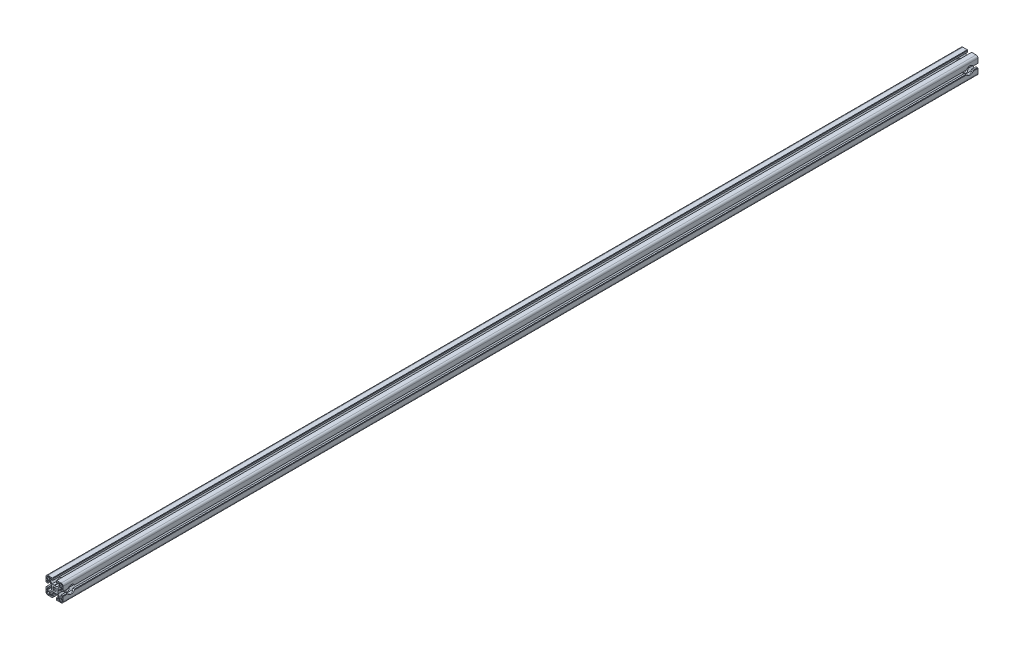
from build123d import *

# Parameters (mm, degrees)
EXTRUDE_1_DEPTH         = 2144
HOLE_WIZARD_19_0_19_1_D = 19


with BuildPart() as part:
    # 草图1 → 凸台-拉伸1 (new body)
    with BuildSketch(Plane.XY):
        with BuildLine():
            Line((-18.9995, -4.100341675), (-18.9995, -5.100341675))
            Line((-18.9995, -5.100341675), (-19.9995, -5.100341675))
            Line((-19.9995, -5.100341675), (-19.9995, -15.500341675))
            ThreePointArc((-19.9995, -15.500341675), (-18.681480515, -18.682322191), (-15.4995, -20.000341675))
            Line((-15.4995, -20.000341675), (-5.0995, -20.000341675))
            Line((-5.0995, -20.000341675), (-5.0995, -19.000341675))
            Line((-5.0995, -19.000341675), (-4.0995, -19.000341675))
            Line((-4.0995, -19.000341675), (-4.0995, -15.500341675))
            Line((-4.0995, -15.500341675), (-6.5995, -15.500341675))
            Line((-6.5995, -15.500341675), (-6.5995, -16.500341675))
            ThreePointArc((-6.5995, -16.500341675), (-6.892393219, -17.207448457), (-7.5995, -17.500341675))
            Line((-7.5995, -17.500341675), (-9.7995, -17.500341675))
            ThreePointArc((-9.7995, -17.500341675), (-10.153053391, -17.353895066), (-10.2995, -17.000341675))
            Line((-10.2995, -17.000341675), (-10.2995, -11.997341675))
            Line((-10.2995, -11.997341675), (-5.9025, -7.600341675))
            Line((-5.9025, -7.600341675), (-0.5195, -7.600341675))
            Line((-0.5195, -7.600341675), (0.0005, -7.300341675))
            Line((0.0005, -7.300341675), (0.5195, -7.600341675))
            Line((0.5195, -7.600341675), (5.9035, -7.600341675))
            Line((5.9035, -7.600341675), (10.3005, -11.997341675))
            Line((10.3005, -11.997341675), (10.3005, -17.000341675))
            ThreePointArc((10.3005, -17.000341675), (10.154053391, -17.353895066), (9.8005, -17.500341675))
            Line((9.8005, -17.500341675), (7.6005, -17.500341675))
            ThreePointArc((7.6005, -17.500341675), (6.893393219, -17.207448457), (6.6005, -16.500341675))
            Line((6.6005, -16.500341675), (6.6005, -15.500341675))
            Line((6.6005, -15.500341675), (4.1005, -15.500341675))
            Line((4.1005, -15.500341675), (4.1005, -19.000341675))
            Line((4.1005, -19.000341675), (5.1005, -19.000341675))
            Line((5.1005, -19.000341675), (5.1005, -20.000341675))
            Line((5.1005, -20.000341675), (15.5005, -20.000341675))
            ThreePointArc((15.5005, -20.000341675), (18.682480515, -18.682322191), (20.0005, -15.500341675))
            Line((20.0005, -15.500341675), (20.0005, -5.100341675))
            Line((20.0005, -5.100341675), (19.0005, -5.100341675))
            Line((19.0005, -5.100341675), (19.0005, -4.100341675))
            Line((19.0005, -4.100341675), (15.5005, -4.100341675))
            Line((15.5005, -4.100341675), (15.5005, -6.600341675))
            Line((15.5005, -6.600341675), (16.5005, -6.600341675))
            ThreePointArc((16.5005, -6.600341675), (17.207606781, -6.893234894), (17.5005, -7.600341675))
            Line((17.5005, -7.600341675), (17.5005, -9.800341675))
            ThreePointArc((17.5005, -9.800341675), (17.354053391, -10.153895066), (17.0005, -10.300341675))
            Line((17.0005, -10.300341675), (11.9975, -10.300341675))
            Line((11.9975, -10.300341675), (7.6005, -5.903341675))
            Line((7.6005, -5.903341675), (7.6005, -0.520341675))
            Line((7.6005, -0.520341675), (7.3005, -0.000341675))
            Line((7.3005, -0.000341675), (7.6005, 0.519658325))
            Line((7.6005, 0.519658325), (7.6005, 5.902658325))
            Line((7.6005, 5.902658325), (11.9975, 10.299658325))
            Line((11.9975, 10.299658325), (17.0005, 10.299658325))
            ThreePointArc((17.0005, 10.299658325), (17.354053391, 10.153211715), (17.5005, 9.799658325))
            Line((17.5005, 9.799658325), (17.5005, 7.599658325))
            ThreePointArc((17.5005, 7.599658325), (17.207606781, 6.892551543), (16.5005, 6.599658325))
            Line((16.5005, 6.599658325), (15.5005, 6.599658325))
            Line((15.5005, 6.599658325), (15.5005, 4.099658325))
            Line((15.5005, 4.099658325), (19.0005, 4.099658325))
            Line((19.0005, 4.099658325), (19.0005, 5.099658325))
            Line((19.0005, 5.099658325), (20.0005, 5.099658325))
            Line((20.0005, 5.099658325), (20.0005, 15.499658325))
            ThreePointArc((20.0005, 15.499658325), (18.682480515, 18.68163884), (15.5005, 19.999658325))
            Line((15.5005, 19.999658325), (5.1005, 19.999658325))
            Line((5.1005, 19.999658325), (5.1005, 18.999658325))
            Line((5.1005, 18.999658325), (4.1005, 18.999658325))
            Line((4.1005, 18.999658325), (4.1005, 15.499658325))
            Line((4.1005, 15.499658325), (6.6005, 15.499658325))
            ThreePointArc((6.6005, 15.499658325), (6.393348977, 15.999658325), (6.6005, 16.499658325))
            ThreePointArc((6.6005, 16.499658325), (6.893393219, 17.206765106), (7.6005, 17.499658325))
            Line((7.6005, 17.499658325), (9.8005, 17.499658325))
            ThreePointArc((9.8005, 17.499658325), (10.154053391, 17.353211715), (10.3005, 16.999658325))
            Line((10.3005, 16.999658325), (10.3005, 11.996658325))
            Line((10.3005, 11.996658325), (5.9035, 7.599658325))
            Line((5.9035, 7.599658325), (0.5195, 7.599658325))
            Line((0.5195, 7.599658325), (0.0005, 7.299658325))
            Line((0.0005, 7.299658325), (-0.5195, 7.599658325))
            Line((-0.5195, 7.599658325), (-5.9025, 7.599658325))
            Line((-5.9025, 7.599658325), (-10.2995, 11.996658325))
            Line((-10.2995, 11.996658325), (-10.2995, 16.999658325))
            ThreePointArc((-10.2995, 16.999658325), (-10.153053391, 17.353211715), (-9.7995, 17.499658325))
            Line((-9.7995, 17.499658325), (-7.5995, 17.499658325))
            ThreePointArc((-7.5995, 17.499658325), (-6.892393219, 17.206765106), (-6.5995, 16.499658325))
            Line((-6.5995, 16.499658325), (-6.5995, 15.499658325))
            Line((-6.5995, 15.499658325), (-4.0995, 15.499658325))
            Line((-4.0995, 15.499658325), (-4.0995, 18.999658325))
            Line((-4.0995, 18.999658325), (-5.0995, 18.999658325))
            Line((-5.0995, 18.999658325), (-5.0995, 19.999658325))
            Line((-5.0995, 19.999658325), (-15.4995, 19.999658325))
            ThreePointArc((-15.4995, 19.999658325), (-18.681480515, 18.68163884), (-19.9995, 15.499658325))
            Line((-19.9995, 15.499658325), (-19.9995, 5.099658325))
            Line((-19.9995, 5.099658325), (-18.9995, 5.099658325))
            Line((-18.9995, 5.099658325), (-18.9995, 4.099658325))
            Line((-18.9995, 4.099658325), (-15.4995, 4.099658325))
            Line((-15.4995, 4.099658325), (-15.4995, 6.599658325))
            Line((-15.4995, 6.599658325), (-16.4995, 6.599658325))
            ThreePointArc((-16.4995, 6.599658325), (-17.206606781, 6.892551543), (-17.4995, 7.599658325))
            Line((-17.4995, 7.599658325), (-17.4995, 9.799658325))
            ThreePointArc((-17.4995, 9.799658325), (-17.353053391, 10.153211715), (-16.9995, 10.299658325))
            Line((-16.9995, 10.299658325), (-11.9965, 10.299658325))
            Line((-11.9965, 10.299658325), (-7.5995, 5.902658325))
            Line((-7.5995, 5.902658325), (-7.5995, 0.519658325))
            Line((-7.5995, 0.519658325), (-7.2995, -0.000341675))
            Line((-7.2995, -0.000341675), (-7.5995, -0.520341675))
            Line((-7.5995, -0.520341675), (-7.5995, -5.903341675))
            Line((-7.5995, -5.903341675), (-11.9965, -10.300341675))
            Line((-11.9965, -10.300341675), (-16.9995, -10.300341675))
            ThreePointArc((-16.9995, -10.300341675), (-17.353053391, -10.153895066), (-17.4995, -9.800341675))
            Line((-17.4995, -9.800341675), (-17.4995, -7.600341675))
            ThreePointArc((-17.4995, -7.600341675), (-17.206606781, -6.893234894), (-16.4995, -6.600341675))
            Line((-16.4995, -6.600341675), (-15.4995, -6.600341675))
            Line((-15.4995, -6.600341675), (-15.4995, -4.100341675))
            Line((-15.4995, -4.100341675), (-18.9995, -4.100341675))
        make_face()
        with BuildLine():
            Line((15.5005, -18.000341675), (11.8005, -18.000341675))
            Line((11.8005, -18.000341675), (11.8005, -11.800341675))
            Line((11.8005, -11.800341675), (18.0005, -11.800341675))
            Line((18.0005, -11.800341675), (18.0005, -15.500341675))
            ThreePointArc((18.0005, -15.500341675), (17.268266953, -17.268108628), (15.5005, -18.000341675))
        make_face(mode=Mode.SUBTRACT)
        with BuildLine():
            Line((18.0005, 11.799658325), (11.8005, 11.799658325))
            Line((11.8005, 11.799658325), (11.8005, 17.999658325))
            Line((11.8005, 17.999658325), (15.5005, 17.999658325))
            ThreePointArc((15.5005, 17.999658325), (17.268266953, 17.267425278), (18.0005, 15.499658325))
            Line((18.0005, 15.499658325), (18.0005, 11.799658325))
        make_face(mode=Mode.SUBTRACT)
        with BuildLine():
            Line((-1.8145, -2.875341675), (-3.004391671, -4.066450004))
            Line((-3.004391671, -4.066450004), (-4.065608329, -3.005233346))
            Line((-4.065608329, -3.005233346), (-2.8745, -1.815341675))
            ThreePointArc((-2.8745, -1.815341675), (-3.399473913, -0.000341675), (-2.8745, 1.814658325))
            Line((-2.8745, 1.814658325), (-4.064391671, 3.005766654))
            Line((-4.064391671, 3.005766654), (-3.004391671, 4.065766654))
            Line((-3.004391671, 4.065766654), (-1.8145, 2.874658325))
            ThreePointArc((-1.8145, 2.874658325), (0, 3.399316649), (1.8145, 2.874658325))
            Line((1.8145, 2.874658325), (3.0055, 4.065658325))
            Line((3.0055, 4.065658325), (4.066608329, 3.004549996))
            Line((4.066608329, 3.004549996), (2.8755, 1.814658325))
            ThreePointArc((2.8755, 1.814658325), (3.400473913, -0.000341675), (2.8755, -1.815341675))
            Line((2.8755, -1.815341675), (4.066608329, -3.005233346))
            Line((4.066608329, -3.005233346), (3.0055, -4.066341675))
            Line((3.0055, -4.066341675), (1.8145, -2.875341675))
            ThreePointArc((1.8145, -2.875341675), (0, -3.4), (-1.8145, -2.875341675))
        make_face(mode=Mode.SUBTRACT)
        with BuildLine():
            Line((-17.9995, -15.500341675), (-17.9995, -11.800341675))
            Line((-17.9995, -11.800341675), (-11.7995, -11.800341675))
            Line((-11.7995, -11.800341675), (-11.7995, -18.000341675))
            Line((-11.7995, -18.000341675), (-15.4995, -18.000341675))
            ThreePointArc((-15.4995, -18.000341675), (-17.267266953, -17.268108628), (-17.9995, -15.500341675))
        make_face(mode=Mode.SUBTRACT)
        with BuildLine():
            Line((-11.7995, 17.999658325), (-11.7995, 11.799658325))
            Line((-11.7995, 11.799658325), (-17.9995, 11.799658325))
            Line((-17.9995, 11.799658325), (-17.9995, 15.499658325))
            ThreePointArc((-17.9995, 15.499658325), (-17.267266953, 17.267425278), (-15.4995, 17.999658325))
            Line((-15.4995, 17.999658325), (-11.7995, 17.999658325))
        make_face(mode=Mode.SUBTRACT)
    extrude(amount=-EXTRUDE_1_DEPTH)

    # Ø19.0 (19) 直径孔1 (through all)
    with Locations(Plane(origin=(20.0005, 0, 0), x_dir=(0, 0, -1), z_dir=(1, 0, 0))):
        with Locations((18.999999997, -0.000341675), (2125, -0.000341675)):
            Hole(HOLE_WIZARD_19_0_19_1_D / 2)


solid = part.part
